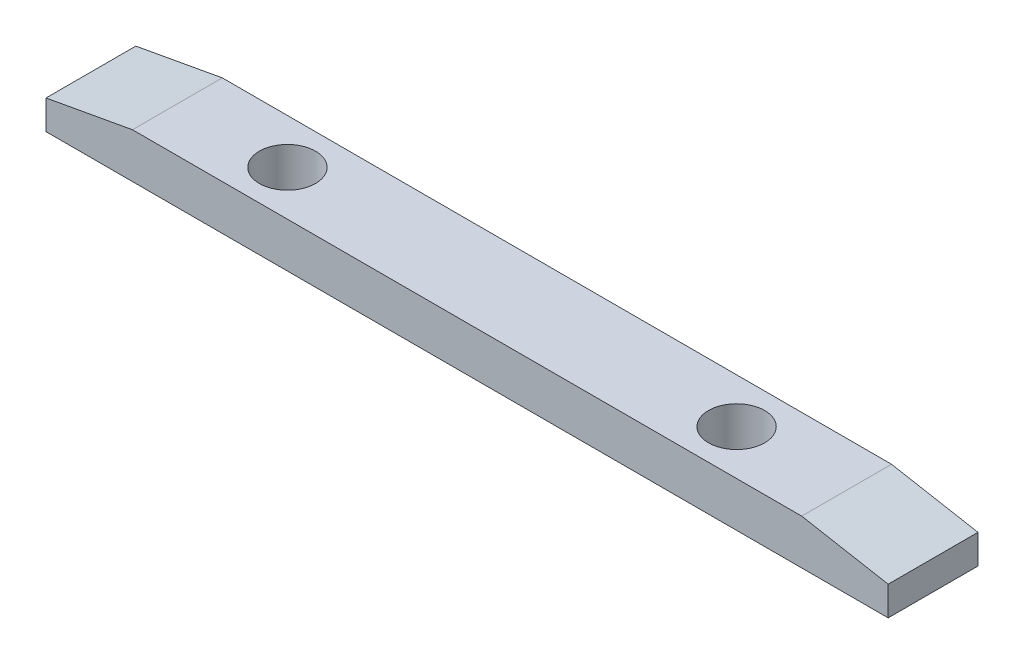
from build123d import *

# Parameters (mm, degrees)
SKETCH_1_W                = 100
SKETCH_1_H                = 136
EXTRUDE_1_DEPTH           = 4
SKETCH_3_W                = 75
SKETCH_3_H                = 15
EXTRUDE_2_DEPTH           = 4
CHAMFER_2_SIZE            = 7.7
CHAMFER_2_SIZE2           = 1.4
CHAMFER_3_SIZE            = 1.4
CHAMFER_3_SIZE2           = 7.7
FILLET_1_R                = 5
CHAMFER_4_SIZE            = 3
HOLE_WIZARD_M4_1_D        = 3.3
HOLE_WIZARD_M4_1_DEPTH    = 11.5
HOLE_WIZARD_M4_1_TIP      = 0.991420021
SKETCH_8_W                = 362.353371429
SKETCH_8_H                = 115.701942857
CUT_EXTRUDE_4_DEPTH       = 114.877126764
CHAMFER_5_SIZE            = 3
HOLE_WIZARD_1_D           = 4.5
HOLE_WIZARD_1_CBORE_D     = 8
HOLE_WIZARD_1_CBORE_DEPTH = 5
CHAMFER_6_SIZE            = 3
SKETCH_14_W               = 127.06003401
SKETCH_14_H               = 84.591980831
CUT_EXTRUDE_5_DEPTH       = 43
SKETCH_15_R               = 2.5
CUT_EXTRUDE_6_DEPTH       = 16.5


with BuildPart() as part:
    # 草图1 → 凸台-拉伸1 (new, symmetric)
    with BuildSketch(Plane.XY):
        with Locations((0, -34)):
            Rectangle(SKETCH_1_W, SKETCH_1_H)
    extrude(amount=EXTRUDE_1_DEPTH, both=True)

    # 草图3 → 凸台-拉伸2 (add, symmetric)
    with BuildSketch(Plane.XY):
        with Locations((0, 41.5)):
            Rectangle(SKETCH_3_W, SKETCH_3_H)
    extrude(amount=EXTRUDE_2_DEPTH, both=True)

    # 倒角2
    chamfer_2_edges = [part.edges().sort_by_distance(p)[0] for p in [
        (-37.5, 49, 0),
    ]]
    chamfer_2_side = [part.faces().sort_by_distance(p)[0] for p in [
        (0, 49, 0),
    ]]
    chamfer(chamfer_2_edges, length=CHAMFER_2_SIZE, length2=CHAMFER_2_SIZE2, reference=chamfer_2_side[0])

    # 倒角3
    chamfer_3_edges = [part.edges().sort_by_distance(p)[0] for p in [
        (37.5, 49, 0),
    ]]
    chamfer_3_side = [part.faces().sort_by_distance(p)[0] for p in [
        (37.5, 41.5, 0),
    ]]
    chamfer(chamfer_3_edges, length=CHAMFER_3_SIZE, length2=CHAMFER_3_SIZE2, reference=chamfer_3_side[0])

    # 圆角1
    fillet_1_edges = [part.edges().sort_by_distance(p)[0] for p in [
        (-37.5, 34, 0),
        (37.5, 34, 0),
    ]]
    fillet(fillet_1_edges, radius=FILLET_1_R)

    # 倒角4
    chamfer_4_edges = [part.edges().sort_by_distance(p)[0] for p in [
        (50, -102, 0),
        (-50, -102, 0),
    ]]
    chamfer(chamfer_4_edges, length=CHAMFER_4_SIZE)

    # M4 螺纹孔1
    with Locations(Plane(origin=(0, 49, 0), x_dir=(1, 0, 0), z_dir=(0, 1, 0))):
        with Locations((-20, 0), (20, 0)):
            Hole(HOLE_WIZARD_M4_1_D / 2, depth=HOLE_WIZARD_M4_1_DEPTH)
            with Locations((0, 0, -(HOLE_WIZARD_M4_1_DEPTH + HOLE_WIZARD_M4_1_TIP / 2))):  # 118° drill point
                Cone(0, HOLE_WIZARD_M4_1_D / 2, HOLE_WIZARD_M4_1_TIP, mode=Mode.SUBTRACT)

    # 草图8 → 切除-拉伸4 (cut, through all)
    with BuildSketch(Plane(origin=(0, 0, -4), x_dir=(-1, 0, 0), z_dir=(0, 0, -1))):
        with Locations((78.704228572, -69.850971429)):
            Rectangle(SKETCH_8_W, SKETCH_8_H)
    extrude(amount=-CUT_EXTRUDE_4_DEPTH, mode=Mode.SUBTRACT)

    # 倒角5
    chamfer_5_edges = [part.edges().sort_by_distance(p)[0] for p in [
        (-50, -12, 0),
        (50, -12, 0),
    ]]
    chamfer(chamfer_5_edges, length=CHAMFER_5_SIZE)

    # 打孔尺寸(%根据)开槽圆柱头螺钉的类型1 (through all)
    with Locations(Plane.XY.offset(4)):
        with Locations((-43.15, -3), (43.15, -3), (-45, 29), (45, 29)):
            CounterBoreHole(HOLE_WIZARD_1_D / 2, HOLE_WIZARD_1_CBORE_D / 2, HOLE_WIZARD_1_CBORE_DEPTH)

    # 倒角6
    chamfer_6_edges = [part.edges().sort_by_distance(p)[0] for p in [
        (-50, 34, 0),
        (50, 34, 0),
    ]]
    chamfer(chamfer_6_edges, length=CHAMFER_6_SIZE)

    # 草图14 → 切除-拉伸5 (cut)
    with BuildSketch(Plane.XY.offset(4)):
        with Locations((-7.727502701, 2.704009584)):
            Rectangle(SKETCH_14_W, SKETCH_14_H)
    extrude(amount=-CUT_EXTRUDE_5_DEPTH, mode=Mode.SUBTRACT)

    # 草图15 → 切除-拉伸6 (cut)
    with BuildSketch(Plane(origin=(0, 49, 0), x_dir=(1, 0, 0), z_dir=(0, 1, 0))):
        with Locations(Location((-20, 0, 0), (0, 0, 270))):
            Circle(SKETCH_15_R)
        with Locations(Location((20, 0, 0), (0, 0, 270))):
            Circle(SKETCH_15_R)
    extrude(amount=-CUT_EXTRUDE_6_DEPTH, mode=Mode.SUBTRACT)


solid = part.part
